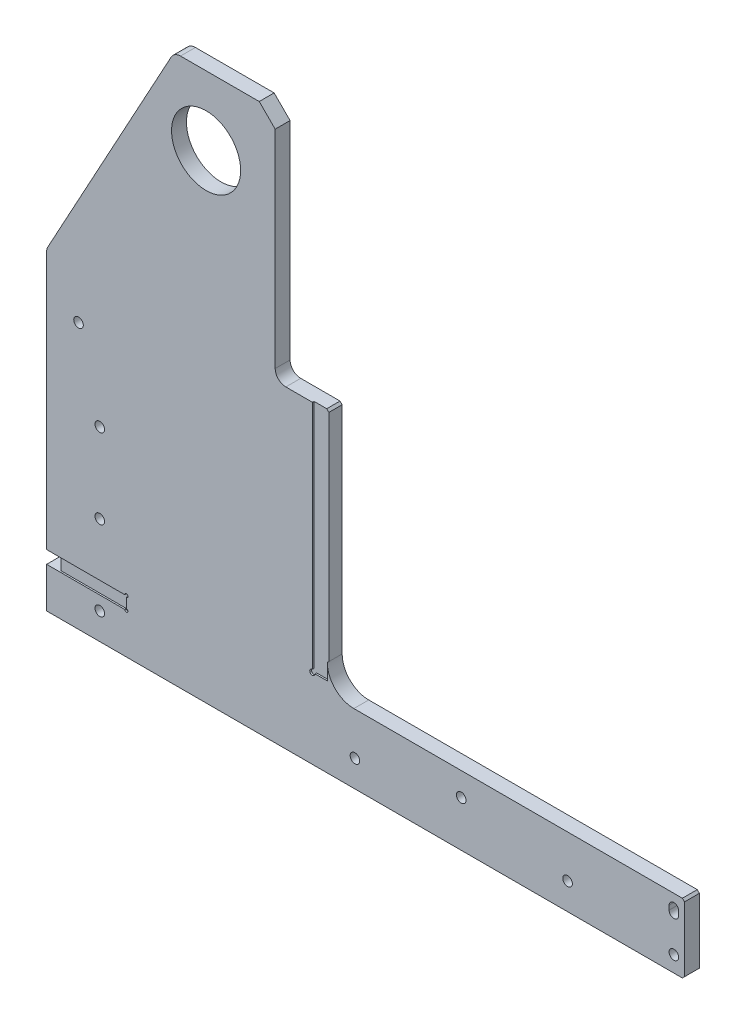
from build123d import *

# Parameters (mm, degrees)
SKETCH_1_W           = 600
SKETCH_1_H           = 515
EXTRUDE_1_DEPTH      = 7
CUT_EXTRUDE_1_REACH  = 397.604
SKETCH_2_R           = 32.5
CUT_EXTRUDE_2_REACH  = 397.604
SKETCH_3_R           = 4.5
SKETCH_4_W           = 150
SKETCH_4_H           = 16
CUT_EXTRUDE_3_DEPTH  = 1.5
SKETCH_5_R           = 2.5
CUT_EXTRUDE_4_DEPTH  = 1.5
SKETCH_6_W           = 75
SKETCH_6_H           = 12
CUT_EXTRUDE_5_DEPTH  = 1.5
SKETCH_7_R           = 1.5
CUT_EXTRUDE_6_DEPTH  = 1.5
CUT_EXTRUDE_7_REACH  = 397.553
SKETCH_8_W           = 12
SKETCH_8_H           = 12
CUT_EXTRUDE_8_REACH  = 397.604
SKETCH_9_R           = 4.5
CUT_EXTRUDE_9_REACH  = 397.604
FILLET_1_R           = 25
SKETCH_11_W          = 14
SKETCH_11_H          = 220
CUT_EXTRUDE_10_DEPTH = 1.5
SKETCH_12_R          = 2.5
CUT_EXTRUDE_11_DEPTH = 1.5
FILLET_2_R           = 10
CHAMFER_2_SIZE       = 2
CHAMFER_3_SIZE       = 2
CUT_EXTRUDE_12_REACH = 397.604
CHAMFER_4_SIZE       = 15
FILLET_3_R           = 10


with BuildPart() as part:
    # 草图1 → 凸台-拉伸1 (new, symmetric)
    with BuildSketch(Plane.XY):
        Rectangle(SKETCH_1_W, SKETCH_1_H)
    extrude(amount=EXTRUDE_1_DEPTH, both=True)

    # 草图2 → 切除-拉伸1 (cut, up to next)
    with BuildSketch(Plane.XY.offset(7), mode=Mode.PRIVATE) as cut_extrude_1_sk1:
        with Locations((-150, 192.5)):
            Circle(SKETCH_2_R)
    cut_extrude_1_tool1 = extrude(cut_extrude_1_sk1.sketch, amount=-CUT_EXTRUDE_1_REACH, mode=Mode.PRIVATE) & part.part
    add(cut_extrude_1_tool1.solids().sort_by_distance((-150, 192.5, 7))[0], mode=Mode.SUBTRACT)

    # 草图3 → 切除-拉伸2 (cut, up to next)
    with BuildSketch(Plane(origin=(0, 0, -7), x_dir=(-1, 0, 0), z_dir=(0, 0, -1)), mode=Mode.PRIVATE) as cut_extrude_2_sk1:
        with Locations((270, -7.5)):
            Circle(SKETCH_3_R)
    cut_extrude_2_tool1 = extrude(cut_extrude_2_sk1.sketch, amount=-CUT_EXTRUDE_2_REACH, mode=Mode.PRIVATE) & part.part
    # 草图3 → 切除-拉伸2 (cut, up to next)
    with BuildSketch(Plane(origin=(0, 0, -7), x_dir=(-1, 0, 0), z_dir=(0, 0, -1)), mode=Mode.PRIVATE) as cut_extrude_2_sk2:
        with Locations((250, -82.5)):
            Circle(SKETCH_3_R)
    cut_extrude_2_tool2 = extrude(cut_extrude_2_sk2.sketch, amount=-CUT_EXTRUDE_2_REACH, mode=Mode.PRIVATE) & part.part
    # 草图3 → 切除-拉伸2 (cut, up to next)
    with BuildSketch(Plane(origin=(0, 0, -7), x_dir=(-1, 0, 0), z_dir=(0, 0, -1)), mode=Mode.PRIVATE) as cut_extrude_2_sk3:
        with Locations((250, -157.5)):
            Circle(SKETCH_3_R)
    cut_extrude_2_tool3 = extrude(cut_extrude_2_sk3.sketch, amount=-CUT_EXTRUDE_2_REACH, mode=Mode.PRIVATE) & part.part
    # 草图3 → 切除-拉伸2 (cut, up to next)
    with BuildSketch(Plane(origin=(0, 0, -7), x_dir=(-1, 0, 0), z_dir=(0, 0, -1)), mode=Mode.PRIVATE) as cut_extrude_2_sk4:
        with Locations((250, -232.5)):
            Circle(SKETCH_3_R)
    cut_extrude_2_tool4 = extrude(cut_extrude_2_sk4.sketch, amount=-CUT_EXTRUDE_2_REACH, mode=Mode.PRIVATE) & part.part
    # 草图3 → 切除-拉伸2 (cut, up to next)
    with BuildSketch(Plane(origin=(0, 0, -7), x_dir=(-1, 0, 0), z_dir=(0, 0, -1)), mode=Mode.PRIVATE) as cut_extrude_2_sk5:
        with Locations((10, -232.5)):
            Circle(SKETCH_3_R)
    cut_extrude_2_tool5 = extrude(cut_extrude_2_sk5.sketch, amount=-CUT_EXTRUDE_2_REACH, mode=Mode.PRIVATE) & part.part
    add(cut_extrude_2_tool1.solids().sort_by_distance((-270, -7.5, -7))[0], mode=Mode.SUBTRACT)
    add(cut_extrude_2_tool2.solids().sort_by_distance((-250, -82.5, -7))[0], mode=Mode.SUBTRACT)
    add(cut_extrude_2_tool3.solids().sort_by_distance((-250, -157.5, -7))[0], mode=Mode.SUBTRACT)
    add(cut_extrude_2_tool4.solids().sort_by_distance((-250, -232.5, -7))[0], mode=Mode.SUBTRACT)
    add(cut_extrude_2_tool5.solids().sort_by_distance((-10, -232.5, -7))[0], mode=Mode.SUBTRACT)

    # 草图4 → 切除-拉伸3 (cut)
    with BuildSketch(Plane(origin=(0, 0, -7), x_dir=(-1, 0, 0), z_dir=(0, 0, -1))):
        with Locations((131, -92)):
            Rectangle(SKETCH_4_W, SKETCH_4_H)
        with Locations((131, -148)):
            Rectangle(SKETCH_4_W, SKETCH_4_H)
    extrude(amount=-CUT_EXTRUDE_3_DEPTH, mode=Mode.SUBTRACT)

    # 草图5 → 切除-拉伸4 (cut)
    with BuildSketch(Plane(origin=(0, 0, -7), x_dir=(-1, 0, 0), z_dir=(0, 0, -1))):
        with Locations((206, -84)):
            Circle(SKETCH_5_R)
        with Locations((206, -100)):
            Circle(SKETCH_5_R)
        with Locations((206, -140)):
            Circle(SKETCH_5_R)
        with Locations((206, -156)):
            Circle(SKETCH_5_R)
        with Locations((56, -84)):
            Circle(SKETCH_5_R)
        with Locations((56, -100)):
            Circle(SKETCH_5_R)
        with Locations((56, -140)):
            Circle(SKETCH_5_R)
        with Locations((56, -156)):
            Circle(SKETCH_5_R)
    extrude(amount=-CUT_EXTRUDE_4_DEPTH, mode=Mode.SUBTRACT)

    # 草图6 → 切除-拉伸5 (cut)
    with BuildSketch(Plane.XY.offset(7)):
        with Locations((-262.5, -213.5)):
            Rectangle(SKETCH_6_W, SKETCH_6_H)
    extrude(amount=-CUT_EXTRUDE_5_DEPTH, mode=Mode.SUBTRACT)

    # 草图7 → 切除-拉伸6 (cut)
    with BuildSketch(Plane.XY.offset(7)):
        with Locations((-225, -207.5)):
            Circle(SKETCH_7_R)
        with Locations((-225, -219.5)):
            Circle(SKETCH_7_R)
    extrude(amount=-CUT_EXTRUDE_6_DEPTH, mode=Mode.SUBTRACT)

    # 草图8 → 切除-拉伸7 (cut, up to next)
    with BuildSketch(Plane.XY.offset(5.5), mode=Mode.PRIVATE) as cut_extrude_7_sk1:
        with Locations((-294, -213.5)):
            Rectangle(SKETCH_8_W, SKETCH_8_H)
    cut_extrude_7_tool1 = extrude(cut_extrude_7_sk1.sketch, amount=-CUT_EXTRUDE_7_REACH, mode=Mode.PRIVATE) & part.part
    add(cut_extrude_7_tool1.solids().sort_by_distance((-294, -213.5, 5.5))[0], mode=Mode.SUBTRACT)

    # 草图9 → 切除-拉伸8 (cut, up to next)
    with BuildSketch(Plane(origin=(0, 0, -7), x_dir=(-1, 0, 0), z_dir=(0, 0, -1)), mode=Mode.PRIVATE) as cut_extrude_8_sk1:
        with Locations((-90, -214.5)):
            Circle(SKETCH_9_R)
    cut_extrude_8_tool1 = extrude(cut_extrude_8_sk1.sketch, amount=-CUT_EXTRUDE_8_REACH, mode=Mode.PRIVATE) & part.part
    # 草图9 → 切除-拉伸8 (cut, up to next)
    with BuildSketch(Plane(origin=(0, 0, -7), x_dir=(-1, 0, 0), z_dir=(0, 0, -1)), mode=Mode.PRIVATE) as cut_extrude_8_sk2:
        with Locations((-190, -232.5)):
            Circle(SKETCH_9_R)
    cut_extrude_8_tool2 = extrude(cut_extrude_8_sk2.sketch, amount=-CUT_EXTRUDE_8_REACH, mode=Mode.PRIVATE) & part.part
    # 草图9 → 切除-拉伸8 (cut, up to next)
    with BuildSketch(Plane(origin=(0, 0, -7), x_dir=(-1, 0, 0), z_dir=(0, 0, -1)), mode=Mode.PRIVATE) as cut_extrude_8_sk3:
        with Locations((-290, -242.5)):
            Circle(SKETCH_9_R)
    cut_extrude_8_tool3 = extrude(cut_extrude_8_sk3.sketch, amount=-CUT_EXTRUDE_8_REACH, mode=Mode.PRIVATE) & part.part
    # 草图9 → 切除-拉伸8 (cut, up to next)
    with BuildSketch(Plane(origin=(0, 0, -7), x_dir=(-1, 0, 0), z_dir=(0, 0, -1)), mode=Mode.PRIVATE) as cut_extrude_8_sk4:
        with BuildLine():
            Line((-285.5, -204.5), (-285.5, -208.5))
            ThreePointArc((-285.5, -208.5), (-290, -213), (-294.5, -208.5))
            Line((-294.5, -208.5), (-294.5, -204.5))
            ThreePointArc((-294.5, -204.5), (-290, -200), (-285.5, -204.5))
        make_face()
    cut_extrude_8_tool4 = extrude(cut_extrude_8_sk4.sketch, amount=-CUT_EXTRUDE_8_REACH, mode=Mode.PRIVATE) & part.part
    add(cut_extrude_8_tool1.solids().sort_by_distance((90, -214.5, -7))[0], mode=Mode.SUBTRACT)
    add(cut_extrude_8_tool2.solids().sort_by_distance((190, -232.5, -7))[0], mode=Mode.SUBTRACT)
    add(cut_extrude_8_tool3.solids().sort_by_distance((290, -242.5, -7))[0], mode=Mode.SUBTRACT)
    add(cut_extrude_8_tool4.solids().sort_by_distance((290, -206.5, -7))[0], mode=Mode.SUBTRACT)

    # 草图10 → 切除-拉伸9 (cut, up to next)
    with BuildSketch(Plane(origin=(0, 0, -7), x_dir=(-1, 0, 0), z_dir=(0, 0, -1)), mode=Mode.PRIVATE) as cut_extrude_9_sk1:
        Polygon((-300, 257.5), (-300, -192.5), (36, -192.5), (36, 37.5), (85, 37.5), (85, 257.5), align=None)
    cut_extrude_9_tool1 = extrude(cut_extrude_9_sk1.sketch, amount=-CUT_EXTRUDE_9_REACH, mode=Mode.PRIVATE) & part.part
    add(cut_extrude_9_tool1.solids().sort_by_distance((119.18885, 40.153414, -7))[0], mode=Mode.SUBTRACT)

    # 圆角1
    fillet_1_edges = [part.edges().sort_by_distance(p)[0] for p in [
        (-36, -192.5, 0),
    ]]
    fillet(fillet_1_edges, radius=FILLET_1_R)

    # 草图11 → 切除-拉伸10 (cut)
    with BuildSketch(Plane.XY.offset(7)):
        with Locations((-43, -72.5)):
            Rectangle(SKETCH_11_W, SKETCH_11_H)
    extrude(amount=-CUT_EXTRUDE_10_DEPTH, mode=Mode.SUBTRACT)

    # 草图12 → 切除-拉伸11 (cut)
    with BuildSketch(Plane.XY.offset(7)):
        with Locations((-50, -182.5)):
            Circle(SKETCH_12_R)
    extrude(amount=-CUT_EXTRUDE_11_DEPTH, mode=Mode.SUBTRACT)

    # 圆角2
    fillet_2_edges = [part.edges().sort_by_distance(p)[0] for p in [
        (-85, 37.5, 0),
    ]]
    fillet(fillet_2_edges, radius=FILLET_2_R)

    # 倒角2
    chamfer_2_edges = [part.edges().sort_by_distance(p)[0] for p in [
        (-36, 37.5, -0.75),
    ]]
    chamfer(chamfer_2_edges, length=CHAMFER_2_SIZE)

    # 倒角3
    chamfer_3_edges = [part.edges().sort_by_distance(p)[0] for p in [
        (300, -192.5, 0),
        (300, -257.5, 0),
    ]]
    chamfer(chamfer_3_edges, length=CHAMFER_3_SIZE)

    # 草图13 → 切除-拉伸12 (cut, up to next)
    with BuildSketch(Plane.XY.offset(7), mode=Mode.PRIVATE) as cut_extrude_12_sk1:
        Polygon((-180, 257.5), (-300, 37.5), (-300, 257.5), align=None)
    cut_extrude_12_tool1 = extrude(cut_extrude_12_sk1.sketch, amount=-CUT_EXTRUDE_12_REACH, mode=Mode.PRIVATE) & part.part
    add(cut_extrude_12_tool1.solids().sort_by_distance((-260, 184.166667, 7))[0], mode=Mode.SUBTRACT)

    # 倒角4
    chamfer_4_edges = [part.edges().sort_by_distance(p)[0] for p in [
        (-85, 257.5, 0),
    ]]
    chamfer(chamfer_4_edges, length=CHAMFER_4_SIZE)

    # 圆角3
    fillet_3_edges = [part.edges().sort_by_distance(p)[0] for p in [
        (-180, 257.5, 0),
        (-300, 37.5, 0),
    ]]
    fillet(fillet_3_edges, radius=FILLET_3_R)


solid = part.part
